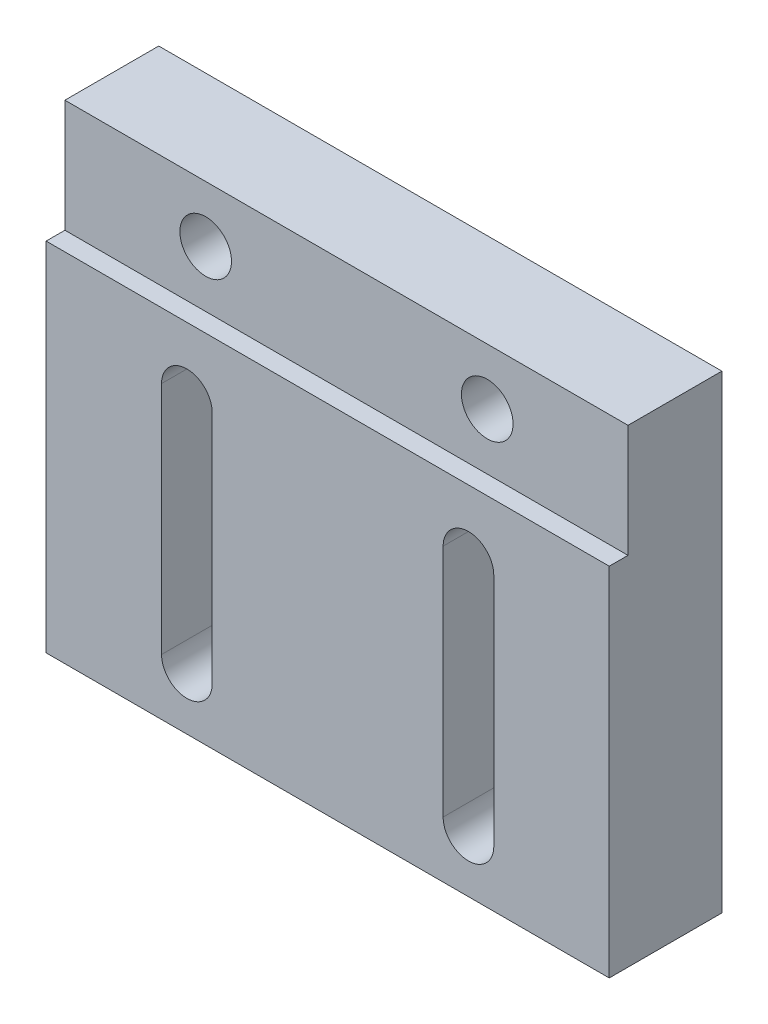
from build123d import *

# Parameters (mm, degrees)
SKETCH_1_W                   = 60
SKETCH_1_H                   = 50
EXTRUDE_1_DEPTH              = 6
SKETCH_2_W                   = 60
SKETCH_2_H                   = 12
CUT_EXTRUDE_1_DEPTH          = 2
CUT_EXTRUDE_2_DEPTH          = 41.853396432
HOLE_WIZARD_M4_1_D           = 5.5
HOLE_WIZARD_M4_1_CBORE_D     = 10
HOLE_WIZARD_M4_1_CBORE_DEPTH = 5.4


with BuildPart() as part:
    # 草图1 → 凸台-拉伸1 (new, symmetric)
    with BuildSketch(Plane.XY):
        Rectangle(SKETCH_1_W, SKETCH_1_H)
    extrude(amount=EXTRUDE_1_DEPTH, both=True)

    # 草图2 → 切除-拉伸1 (cut)
    with BuildSketch(Plane.XY.offset(6)):
        with Locations((0, 19)):
            Rectangle(SKETCH_2_W, SKETCH_2_H)
    extrude(amount=-CUT_EXTRUDE_1_DEPTH, mode=Mode.SUBTRACT)

    # 草图3 → 切除-拉伸2 (cut, through all)
    with BuildSketch(Plane.XY.offset(6)):
        with BuildLine():
            Line((-17.7, -19), (-17.7, 6))
            ThreePointArc((-17.7, 6), (-15, 8.7), (-12.3, 6))
            Line((-12.3, 6), (-12.3, -19))
            ThreePointArc((-12.3, -19), (-15, -21.7), (-17.7, -19))
        make_face()
        with BuildLine():
            Line((12.3, -19), (12.3, 6))
            ThreePointArc((12.3, 6), (15, 8.7), (17.7, 6))
            Line((17.7, 6), (17.7, -19))
            ThreePointArc((17.7, -19), (15, -21.7), (12.3, -19))
        make_face()
    extrude(amount=-CUT_EXTRUDE_2_DEPTH, mode=Mode.SUBTRACT)

    # M4 沉头孔1 (through all)
    with Locations(Plane(origin=(0, 0, -6), x_dir=(-1, 0, 0), z_dir=(0, 0, -1))):
        with Locations((-15, 19), (15, 19)):
            CounterBoreHole(HOLE_WIZARD_M4_1_D / 2, HOLE_WIZARD_M4_1_CBORE_D / 2, HOLE_WIZARD_M4_1_CBORE_DEPTH)


solid = part.part
